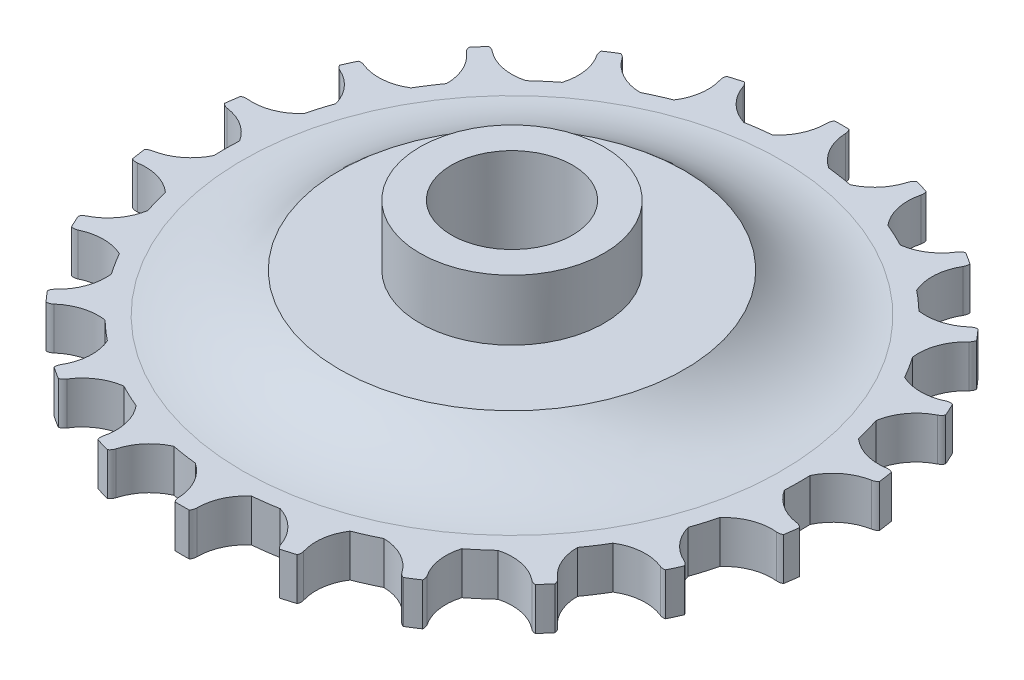
from build123d import *

# Parameters (mm, degrees)
SKETCH1_R           = 10
BOSS_EXTRUDE1_DEPTH = 20
SKETCH4_R           = 15.20255397
SKETCH4_R_2         = 10
BOSS_EXTRUDE4_DEPTH = 10
BOSS_EXTRUDE5_START = 3
SKETCH7_R           = 19.91769717
SKETCH7_R_2         = 10
BOSS_EXTRUDE5_DEPTH = 3


with BuildPart() as part:
    # Sketch1 → Boss-Extrude1 (new body)
    with BuildSketch(Plane(origin=(0, 0, 0), x_dir=(1, 0, 0), z_dir=(0, 1, 0))):
        with BuildLine():
            ThreePointArc((1.498826498, 53.559322248), (-0.039100414, 54.999490299), (-1.499881285, 53.481128534))
            ThreePointArc((-1.499881285, 53.481128534), (-2.210549395, 50.082773833), (-4.293982852, 47.305514597))
            ThreePointArc((-4.293982852, 47.305514597), (-6.390991754, 47.068091361), (-8.475384898, 46.73775616))
            ThreePointArc((-8.475384898, 46.73775616), (-11.670996631, 48.65508342), (-13.651291306, 51.81206159))
            ThreePointArc((-13.651291306, 51.81206159), (-15.5326636, 52.760608635), (-16.506500638, 50.89220166))
            ThreePointArc((-16.506500638, 50.89220166), (-16.230954538, 47.431285859), (-17.447549955, 44.179554101))
            ThreePointArc((-17.447549955, 44.179554101), (-19.392725407, 43.360952495), (-21.299619802, 42.45675678))
            ThreePointArc((-21.299619802, 42.45675678), (-24.905960317, 43.396110951), (-27.695462676, 45.867295841))
            ThreePointArc((-27.695462676, 45.867295841), (-29.767862757, 46.247376238), (-30.175861478, 44.180291275))
            ThreePointArc((-30.175861478, 44.180291275), (-28.936424274, 40.937197189), (-29.187620326, 37.474428878))
            ThreePointArc((-29.187620326, 37.474428878), (-30.823375781, 36.140967135), (-32.398286184, 34.736163466))
            ThreePointArc((-32.398286184, 34.736163466), (-36.123191221, 34.621443659), (-39.495912371, 36.206634565))
            ThreePointArc((-39.495912371, 36.206634565), (-41.591446709, 35.987456463), (-41.400553484, 33.889156442))
            ThreePointArc((-41.400553484, 33.889156442), (-39.297637006, 31.126620266), (-38.563083283, 27.733348296))
            ThreePointArc((-38.563083283, 27.733348296), (-39.756899563, 25.993055557), (-40.872236099, 24.201452772))
            ThreePointArc((-40.872236099, 24.201452772), (-44.413936004, 23.041952903), (-48.096638138, 23.612727086))
            ThreePointArc((-48.096638138, 23.612727086), (-50.045539004, 22.81204699), (-49.271218865, 20.8525237))
            ThreePointArc((-49.271218865, 20.8525237), (-46.475188901, 18.794349686), (-44.814394576, 15.745476772))
            ThreePointArc((-44.814394576, 15.745476772), (-45.469555785, 13.739341204), (-46.034960521, 11.706084306))
            ThreePointArc((-46.034960521, 11.706084306), (-49.106527833, 9.595740159), (-52.800860323, 9.105856889))
            ThreePointArc((-52.800860323, 9.105856889), (-54.44523936, 7.788541139), (-53.150223121, 6.126543502))
            ThreePointArc((-53.150223121, 6.126543502), (-49.887597389, 4.939472669), (-47.435110142, 2.482000361))
            ThreePointArc((-47.435110142, 2.482000361), (-47.498539016, 0.372547137), (-47.468206223, -1.737641491))
            ThreePointArc((-47.468206223, -1.737641491), (-49.820800824, -4.627862385), (-53.227470825, -6.138715679))
            ThreePointArc((-53.227470825, -6.138715679), (-54.434110222, -7.865945995), (-52.723312396, -9.095772814))
            ThreePointArc((-52.723312396, -9.095772814), (-49.258409429, -9.315571048), (-46.212915192, -10.982552957))
            ThreePointArc((-46.212915192, -10.982552957), (-45.6794731, -13.024428483), (-45.055860161, -15.040593909))
            ThreePointArc((-45.055860161, -15.040593909), (-46.498888828, -18.476543041), (-49.341908196, -20.88596601))
            ThreePointArc((-49.341908196, -20.88596601), (-50.013053205, -22.883180966), (-48.025072459, -23.581203711))
            ThreePointArc((-48.025072459, -23.581203711), (-44.638598089, -22.8159226), (-41.246824692, -23.557365151))
            ThreePointArc((-41.246824692, -23.557365151), (-40.15972794, -25.366242366), (-38.993356266, -27.125046859))
            ThreePointArc((-38.993356266, -27.125046859), (-39.409913399, -30.828364065), (-41.458957612, -33.941159589))
            ThreePointArc((-41.458957612, -33.941159589), (-41.540236057, -36.046556705), (-39.436126767, -36.156225726))
            ThreePointArc((-39.436126767, -36.156225726), (-36.402433007, -34.467863795), (-32.939161759, -34.223699721))
            ThreePointArc((-32.939161759, -34.223699721), (-31.386480462, -35.653034152), (-29.771842549, -37.011989831))
            ThreePointArc((-29.771842549, -37.011989831), (-29.128181166, -40.682654375), (-30.217248849, -44.246642274))
            ThreePointArc((-30.217248849, -44.246642274), (-29.702076033, -46.289654798), (-27.65230062, -45.802085363))
            ThreePointArc((-27.65230062, -45.802085363), (-25.217159297, -43.327423653), (-21.962963838, -42.117433676))
            ThreePointArc((-21.962963838, -42.117433676), (-20.070486999, -43.051429147), (-18.138391208, -43.900441505))
            ThreePointArc((-18.138391208, -43.900441505), (-16.486656927, -47.241077976), (-16.527518293, -50.967525147))
            ThreePointArc((-16.527518293, -50.967525147), (-15.457630454, -52.782640354), (-13.628249531, -51.737332438))
            ThreePointArc((-13.628249531, -51.737332438), (-11.988941313, -48.676853325), (-9.207457205, -46.599063637))
            ThreePointArc((-9.207457205, -46.599063637), (-7.128502043, -46.96205339), (-5.035475285, -47.232340495))
            ThreePointArc((-5.035475285, -47.232340495), (-2.509481793, -49.972310394), (-1.498826498, -53.559322248))
            ThreePointArc((-1.498826498, -53.559322248), (0.039100414, -54.999490299), (1.499881285, -53.481128534))
            ThreePointArc((1.499881285, -53.481128534), (2.210549395, -50.082773833), (4.293982852, -47.305514597))
            ThreePointArc((4.293982852, -47.305514597), (6.390991754, -47.068091361), (8.475384898, -46.73775616))
            ThreePointArc((8.475384898, -46.73775616), (11.670996631, -48.65508342), (13.651291306, -51.81206159))
            ThreePointArc((13.651291306, -51.81206159), (15.5326636, -52.760608635), (16.506500638, -50.89220166))
            ThreePointArc((16.506500638, -50.89220166), (16.230954538, -47.431285859), (17.447549955, -44.179554101))
            ThreePointArc((17.447549955, -44.179554101), (19.392725407, -43.360952495), (21.299619802, -42.45675678))
            ThreePointArc((21.299619802, -42.45675678), (24.905960317, -43.396110951), (27.695462676, -45.867295841))
            ThreePointArc((27.695462676, -45.867295841), (29.767862757, -46.247376238), (30.175861478, -44.180291275))
            ThreePointArc((30.175861478, -44.180291275), (28.936424274, -40.937197189), (29.187620326, -37.474428878))
            ThreePointArc((29.187620326, -37.474428878), (30.823375781, -36.140967135), (32.398286184, -34.736163466))
            ThreePointArc((32.398286184, -34.736163466), (36.123191221, -34.621443659), (39.495912371, -36.206634565))
            ThreePointArc((39.495912371, -36.206634565), (41.591446709, -35.987456463), (41.400553484, -33.889156442))
            ThreePointArc((41.400553484, -33.889156442), (39.297637006, -31.126620266), (38.563083283, -27.733348296))
            ThreePointArc((38.563083283, -27.733348296), (39.756899563, -25.993055557), (40.872236099, -24.201452772))
            ThreePointArc((40.872236099, -24.201452772), (44.413936004, -23.041952903), (48.096638138, -23.612727086))
            ThreePointArc((48.096638138, -23.612727086), (50.045539004, -22.81204699), (49.271218865, -20.8525237))
            ThreePointArc((49.271218865, -20.8525237), (46.475188901, -18.794349686), (44.814394576, -15.745476772))
            ThreePointArc((44.814394576, -15.745476772), (45.469555785, -13.739341204), (46.034960521, -11.706084306))
            ThreePointArc((46.034960521, -11.706084306), (49.106527833, -9.595740159), (52.800860323, -9.105856889))
            ThreePointArc((52.800860323, -9.105856889), (54.44523936, -7.788541139), (53.150223121, -6.126543502))
            ThreePointArc((53.150223121, -6.126543502), (49.887597389, -4.939472669), (47.435110142, -2.482000361))
            ThreePointArc((47.435110142, -2.482000361), (47.498539016, -0.372547137), (47.468206223, 1.737641491))
            ThreePointArc((47.468206223, 1.737641491), (49.820800824, 4.627862385), (53.227470825, 6.138715679))
            ThreePointArc((53.227470825, 6.138715679), (54.434110222, 7.865945995), (52.723312396, 9.095772814))
            ThreePointArc((52.723312396, 9.095772814), (49.258409429, 9.315571048), (46.212915192, 10.982552957))
            ThreePointArc((46.212915192, 10.982552957), (45.6794731, 13.024428483), (45.055860161, 15.040593909))
            ThreePointArc((45.055860161, 15.040593909), (46.498888828, 18.476543041), (49.341908196, 20.88596601))
            ThreePointArc((49.341908196, 20.88596601), (50.013053205, 22.883180966), (48.025072459, 23.581203711))
            ThreePointArc((48.025072459, 23.581203711), (44.638598089, 22.8159226), (41.246824692, 23.557365151))
            ThreePointArc((41.246824692, 23.557365151), (40.15972794, 25.366242366), (38.993356266, 27.125046859))
            ThreePointArc((38.993356266, 27.125046859), (39.409913399, 30.828364065), (41.458957612, 33.941159589))
            ThreePointArc((41.458957612, 33.941159589), (41.540236057, 36.046556705), (39.436126767, 36.156225726))
            ThreePointArc((39.436126767, 36.156225726), (36.402433007, 34.467863795), (32.939161759, 34.223699721))
            ThreePointArc((32.939161759, 34.223699721), (31.386480462, 35.653034152), (29.771842549, 37.011989831))
            ThreePointArc((29.771842549, 37.011989831), (29.128181166, 40.682654375), (30.217248849, 44.246642274))
            ThreePointArc((30.217248849, 44.246642274), (29.702076033, 46.289654798), (27.65230062, 45.802085363))
            ThreePointArc((27.65230062, 45.802085363), (25.217159297, 43.327423653), (21.962963838, 42.117433676))
            ThreePointArc((21.962963838, 42.117433676), (20.070486999, 43.051429147), (18.138391208, 43.900441505))
            ThreePointArc((18.138391208, 43.900441505), (16.486656927, 47.241077976), (16.527518293, 50.967525147))
            ThreePointArc((16.527518293, 50.967525147), (15.457630454, 52.782640354), (13.628249531, 51.737332438))
            ThreePointArc((13.628249531, 51.737332438), (11.988941313, 48.676853325), (9.207457205, 46.599063637))
            ThreePointArc((9.207457205, 46.599063637), (7.128502043, 46.96205339), (5.035475285, 47.232340495))
            ThreePointArc((5.035475285, 47.232340495), (2.509481793, 49.972310394), (1.498826498, 53.559322248))
        make_face()
        with Locations(Location((0, 0, 0), (0, 0, 270))):
            Circle(SKETCH1_R, mode=Mode.SUBTRACT)
    extrude(amount=BOSS_EXTRUDE1_DEPTH)

    # Sketch4 → Boss-Extrude4 (add)
    with BuildSketch(Plane(origin=(0, 20, 0), x_dir=(1, 0, 0), z_dir=(0, 1, 0))):
        with Locations(Location((0, 0, 0), (0, 0, 90))):
            Circle(SKETCH4_R)
        with Locations(Location((0, 0, 0), (0, 0, 270))):
            Circle(SKETCH4_R_2, mode=Mode.SUBTRACT)
    extrude(amount=BOSS_EXTRUDE4_DEPTH)

    # Sketch6 → Cut-Revolve1 (revolve, cut)
    with BuildSketch(Plane.XY, mode=Mode.PRIVATE) as cut_revolve1_sk:
        with BuildLine():
            Line((-54.455447141, 13.5), (-54.455447141, 6.5))
            Line((-54.455447141, 6.5), (-44.455447141, 6.5))
            ThreePointArc((-44.455447141, 6.5), (-35.820489121, 4.812973587), (-28.455447141, 0))
            Line((-28.455447141, 0), (-62.695803054, 0))
            Line((-62.695803054, 0), (-62.695803054, 20))
            Line((-62.695803054, 20), (-28.455447141, 20))
            ThreePointArc((-28.455447141, 20), (-35.820489121, 15.187026413), (-44.455447141, 13.5))
            Line((-44.455447141, 13.5), (-54.455447141, 13.5))
        make_face()
    revolve(cut_revolve1_sk.sketch.rotate(Axis((0, 30, 0), (0, -1, 0)), 270), axis=Axis((0, 30, 0), (0, -1, 0)), mode=Mode.SUBTRACT)

    # Sketch7 → Boss-Extrude5 (add)
    with BuildSketch(Plane.XZ.offset(BOSS_EXTRUDE5_START)):
        with Locations(Location((0, 0, 0), (0, 0, 270))):
            Circle(SKETCH7_R)
        with Locations(Location((0, 0, 0), (0, 0, 270))):
            Circle(SKETCH7_R_2, mode=Mode.SUBTRACT)
    extrude(amount=-BOSS_EXTRUDE5_DEPTH)


solid = part.part
